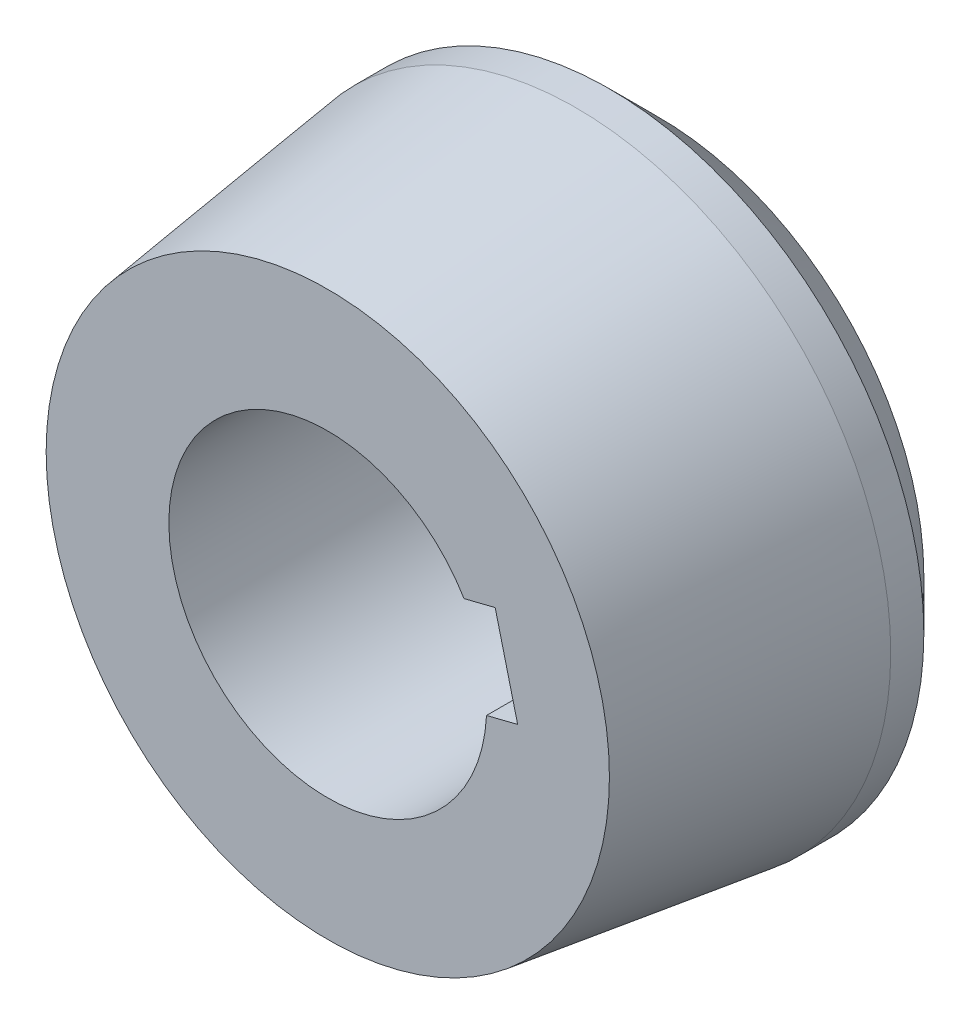
SolidWorks part; units mm, degrees
ref_plane "Front Plane" through (0, 0, 0) normal (0, 0, 1) x (1, 0, 0)
ref_plane "Top Plane" through (0, 0, 0) normal (0, 1, 0) x (1, 0, 0)
ref_plane "Right Plane" through (0, 0, 0) normal (1, 0, 0) x (0, 0, -1)
ref_plane "Plane1" through (0, 234.744, 0) normal (0, 1, 0) x (1, 0, 0)
sketch "Sketch1" plane through (0, 234.744, 0) normal (0, 1, 0) x (1, 0, 0)
  line L0 (561.2306, 824.9984) -> (521.2306, 824.9984)
  line L1 (521.2306, 824.9984) -> (521.2306, 774.9984)
  line L2 (521.2306, 774.9984) -> (563.7556, 774.9984)
  line L3 (563.7556, 774.9984) -> (568.7306, 812.4984)
  line L4 (568.7306, 812.4984) -> (568.7306, 817.4984)
  line L5 (568.7306, 817.4984) -> (561.2306, 824.9984)
  line L6 (521.2306, 824.9984) -> (521.2306, 774.9984) construction
  dimension "D1" = 40
  dimension "D2" = 42.525
  dimension "D3" = 47.5
  dimension "D4" = 37.5
  dimension "D5" = 42.5
  dimension "D6" = 50
revolve "Revolve1" add sketch "Sketch1" angle 360 about L6
sketch "Sketch2" plane through (0, 0, -774.9984) normal (0, 0, 1) x (1, 0, 0)
  line L0 (549.8983, 234.6929) -> (546.5041, 248.2752)
  line L1 (546.5041, 248.2752) -> (541.8051, 247.1009)
  line L2 (545.1993, 233.5186) -> (549.8983, 234.6929)
  arc A0 (541.8051, 247.1009) -> (545.1993, 233.5186) centre (521.2306, 234.744) cw
  circle A1 centre (521.2306, 234.744) radius 42.525 construction
  dimension "D1" = 24
  dimension "D2" = 20.5744
  dimension "D3" = 23.9687
  dimension "D4" = 25.2734
  dimension "D5" = 28.6677
  dimension "D6" = 12.3569
  dimension "D7" = 13.5312
  dimension "D8" = 0.0511
  dimension "D9" = 1.2254
extrude "Cut-Extrude1" cut sketch "Sketch2" against normal through all
ref_plane "Plane2" through (0, 234.744, 0) normal (0, -1, 0) x (1, 0, 0)
sketch "Sketch3" plane through (0, 234.744, 0) normal (0, -1, 0) x (1, 0, 0)
  line L0 (545.2306, -774.9984) -> (521.2306, -774.9984)
  line L1 (521.2306, -774.9984) -> (521.2306, -824.9984)
  line L2 (521.2306, -824.9984) -> (545.2306, -824.9984)
  line L3 (545.2306, -824.9984) -> (545.2306, -774.9984)
  line L4 (521.2306, -774.9984) -> (521.2306, -824.9984) construction
  dimension "D1" = 24
  dimension "D2" = 50
revolve "Cut-Revolve1" cut sketch "Sketch3" angle 360 about L4
